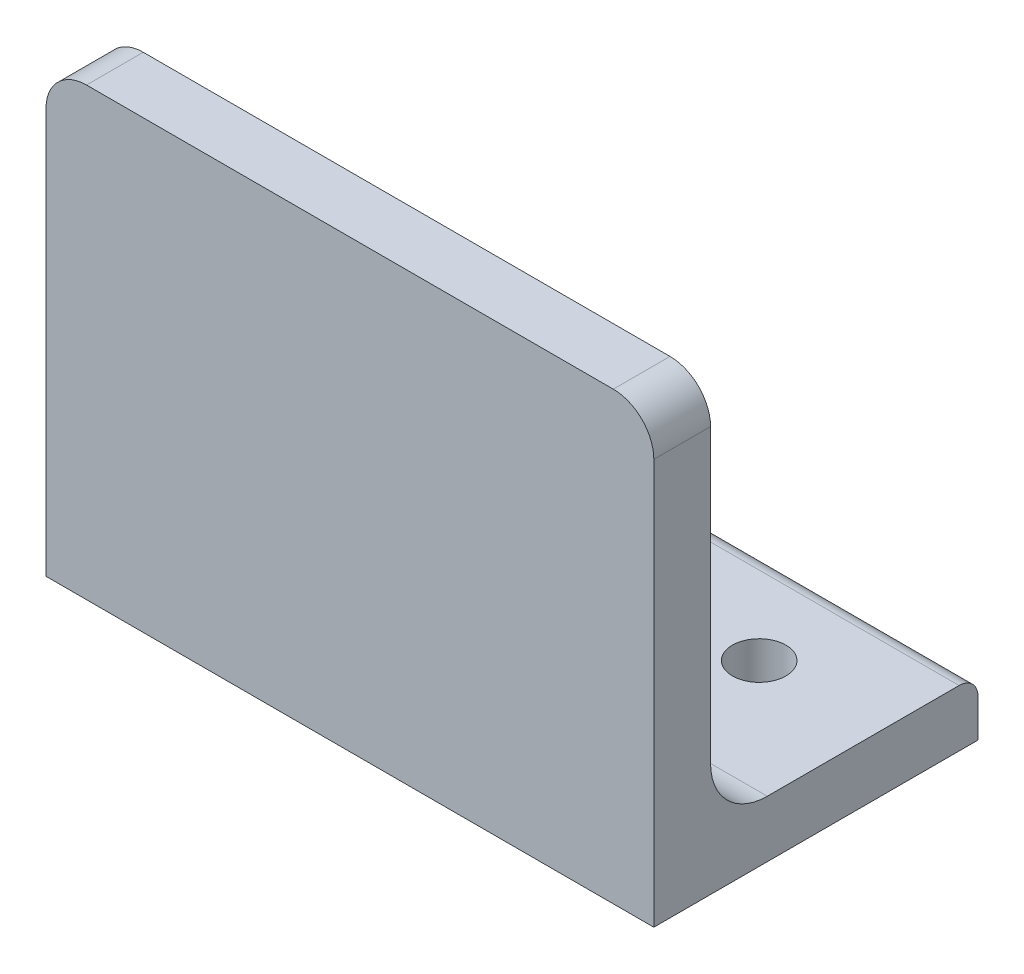
SolidWorks part; units mm, degrees
material "Q235"
ref_plane "Front Plane" through (0, 0, 0) normal (0, 0, 1) x (1, 0, 0)
ref_plane "Top Plane" through (0, 0, 0) normal (0, 1, 0) x (1, 0, 0)
ref_plane "Right Plane" through (0, 0, 0) normal (1, 0, 0) x (0, 0, -1)
sketch3d "3DSketch1"
  line L0 (0, 0, 0) -> (75, 0, 0)
  dimension "D1" = 75
other "Unequal Angle Steel 6.3-4(1)"
ref_plane "Plane1" through (0, 0, 0) normal (1, 0, 0) x (0, 1, 0)
sketch "Sketch11" plane through (0, 0, 0) normal (1, 0, 0) x (0, 1, 0)
  line L0 (63, 0) -> (0, 0)
  line L1 (0, 0) -> (0, -40)
  line L2 (60.6667, -7) -> (14, -7)
  line L3 (7, -14) -> (7, -37.6667)
  line L4 (63, 0) -> (63, -4.6667)
  line L5 (0, -40) -> (4.6667, -40)
  arc A0 (63, -4.6667) -> (60.6667, -7) centre (60.6667, -4.6667) cw
  arc A1 (4.6667, -40) -> (7, -37.6667) centre (4.6667, -37.6667) ccw
  arc A2 (14, -7) -> (7, -14) centre (14, -14) ccw
  point P2 (0, -20)
  point P13 (31.5, 0)
  point P14 (0, 0)
  dimension "r1" = 2.3333
  dimension "r" = 7
  dimension "a" = 63
  dimension "d" = 7
  dimension "b" = 40
hole_wizard "M6 Clearance Hole1" positions "Sketch5" profile "Sketch6" hole size "M6" standard "GB"
sketch "Sketch5" plane through (0, 0, 0) normal (0, 1, 0) x (1, 0, 0)
  line L0 (75, 0) -> (0, 0) construction
  line L3 (0, 37.6667) -> (0, 14) construction
  line L4 (75, 37.6667) -> (75, 14) construction
  point P0 (15, 28)
  point P2 (60, 28)
  dimension "D1" = 28
  dimension "D2" = 15
  dimension "D3" = 15
sketch "Sketch6" plane through (15, 0, -28) normal (1, 0, 0) x (0, 0, -1)
  line L0 (0, 0) -> (0, 21.9828)
  line L1 (0, 21.9828) -> (3.3, 20)
  line L2 (3.3, 20) -> (3.3, 0)
  line L5 (3.3, 0) -> (0, 0)
  line L10 (0, 21.9828) -> (-3.3, 20) construction
  line L11 (0, -6.35) -> (0, 107.95) construction
  dimension "孔直径" = 6.6
  dimension "孔深度" = 20
  dimension "导头角度" = 118
sketch "Sketch8" plane through (75, 0, 0) normal (1, 0, 0) x (0, 0, -1)
  line L0 (7, 14) -> (7, 60.6667) construction
  line L1 (-7, 71) -> (7, 71)
  line L2 (-7, 71) -> (-7, 55)
  line L3 (-7, 55) -> (7, 55)
  line L4 (7, 71) -> (7, 55)
  line L5 (-7, 71) -> (7, 55) construction
  line L6 (-7, 55) -> (7, 71) construction
  line L7 (0, 0) -> (40, 0) construction
  point P0 (0, 63)
  dimension "D1" = 55
extrude "Cut-Extrude1" cut sketch "Sketch8" against normal through all both and the other way through all
fillet "Fillet1" radius 5 2 edges at (0, 55, -3.5) (75, 55, -3.5)
